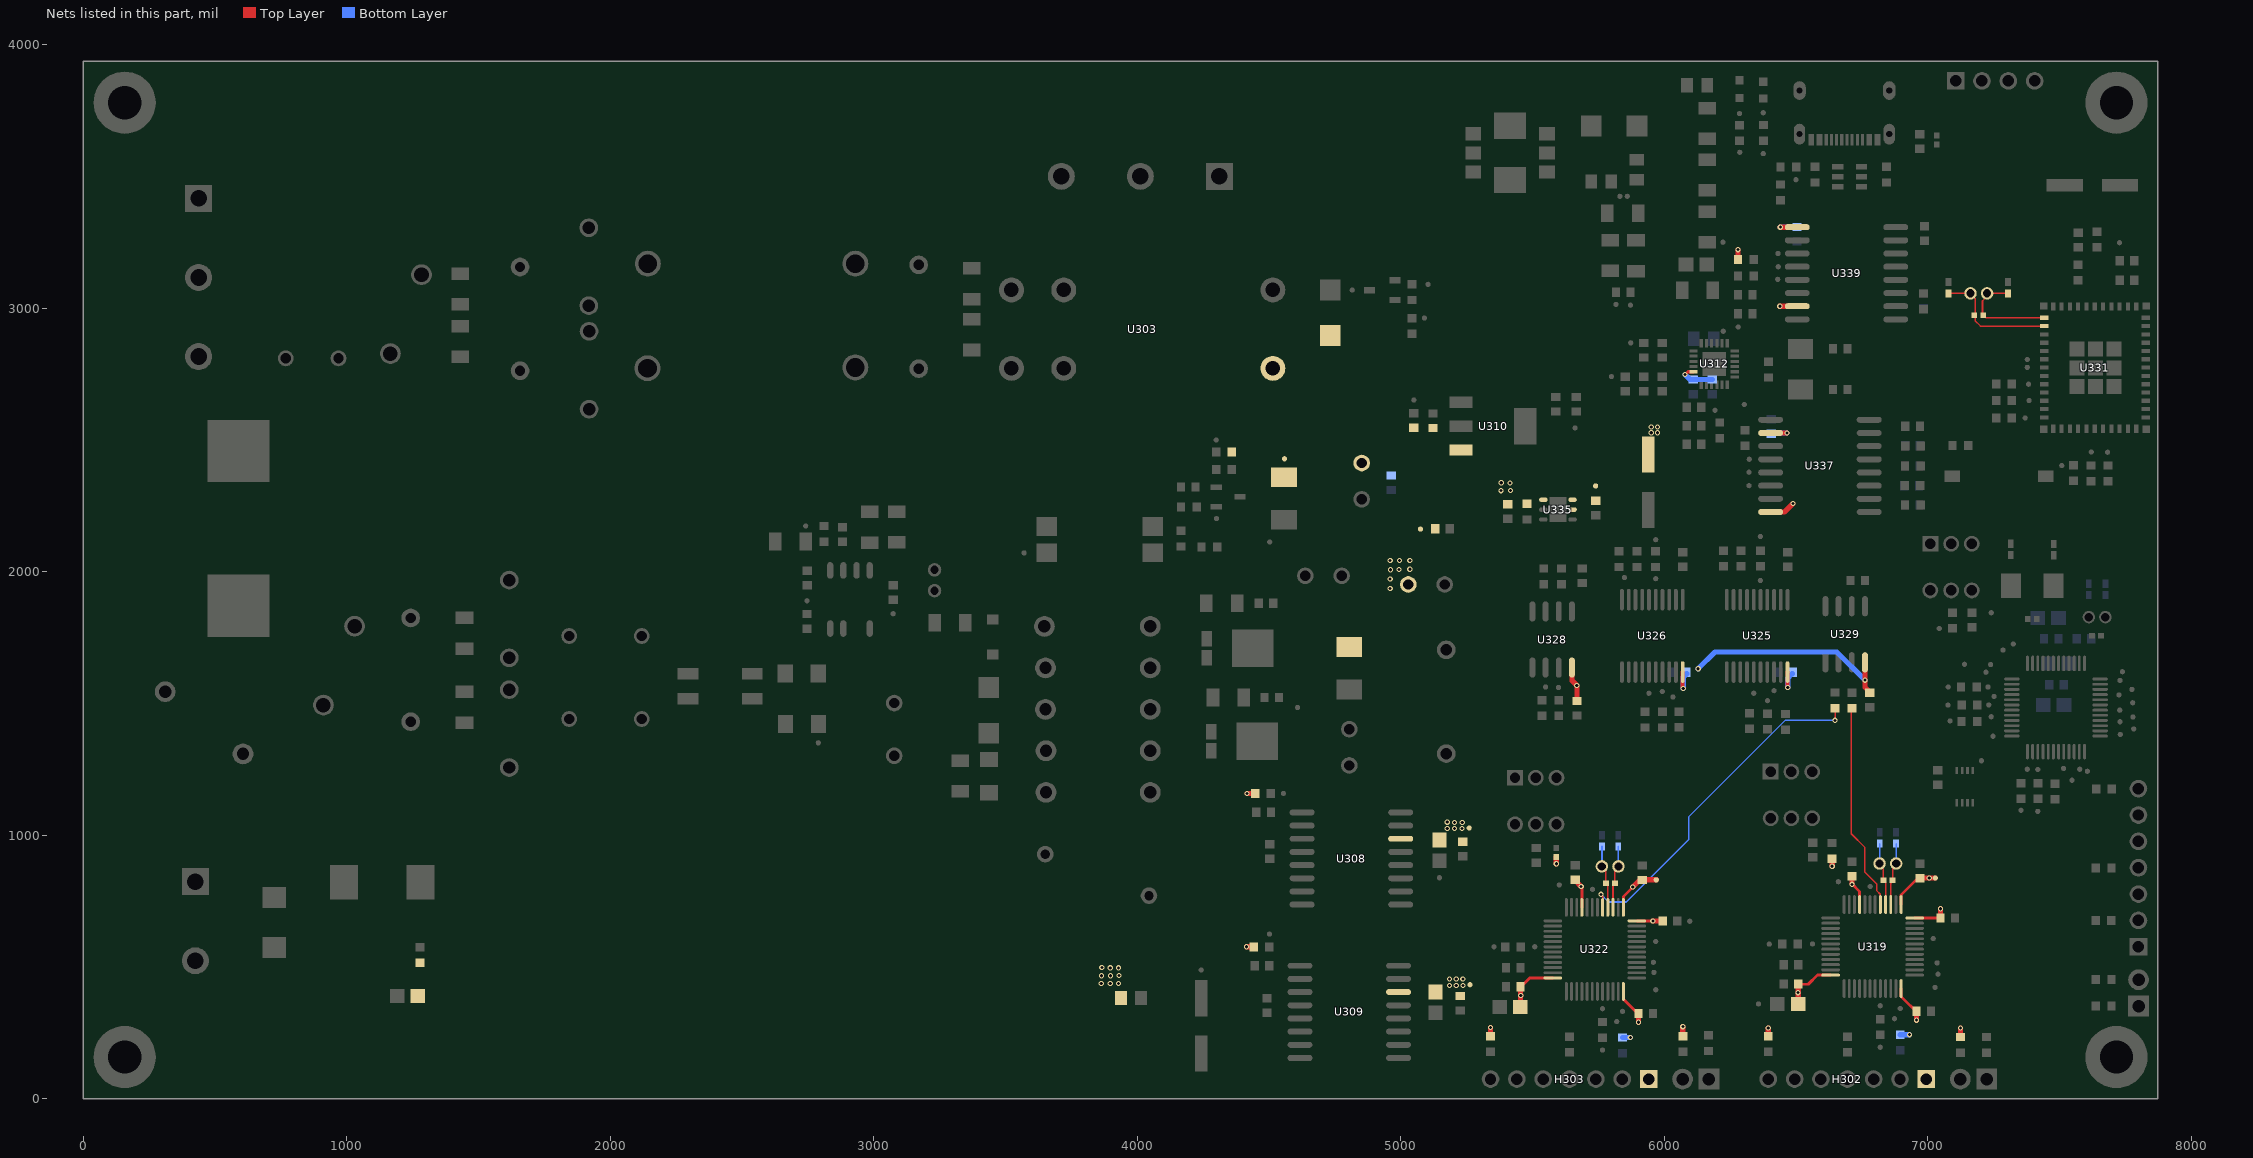
[diagram p0: the nets of this part, all layers, seen from the top]
# Altium PCB MISC84429.PcbDoc (part 5 of 5)
Units mil, origin at the board's own origin, x right, y up, seen from the top; angles counter-clockwise.
Board outline 7874.02 x 3937.01 mil, 4 copper layers (Top Layer, GND, POWER, Bottom Layer); 424 components, 202 nets, 1144 pads, 784 vias.

## Via types
v1: diameter 20, hole 12, Top Layer to Bottom Layer, tented both sides, 695 vias
v2: diameter 20, hole 12, Top Layer to Bottom Layer, 87 vias
v3: diameter 30, hole 15, Top Layer to Bottom Layer, tented both sides, 2 vias

## Nets (pads, with @x,y where several pads share a name; then routed paths per layer and width w, separated by ;. In a path a pad name is that pad's centre, name@x,y a point inside that pad or via, vN(x,y) a via of type N, cw(c..) or ccw(c..) an arc to the next point about the centre after c; other vN are vias at no path point) (continued)
VCC_3V3_HOT: C345.1 C346.1 C347.1 C414.2 C416.1 C418.1 R336.2 TP326.1 U312.17 U335.2 U335.3 U337.10 U337.16 U339.1 U339.7 | length 589.9
  Top Layer w12: v1(6079,2748) 6080,2748 6090.47,2758.47 U312.17@6111.58,2758.47
  Top Layer w20: R336.2@6280.34,3184 v1(6280.34,3221.66) ; U337.16@6403.98,2226 6457,2226 v2(6489,2258) ; U337.10@6403.98,2526 v2(6466,2526) ; v2(6439,3007) U339.7@6504.98,3007 ; v2(6441,3307) U339.1@6504.98,3307
  Bottom Layer w20: v1(6079,2748) 6098.44,2728.56 C346.1@6111,2728.56 C345.1@6183,2728.56 ; C416.1@6411,2526 v2(6466,2526) ; v2(6441,3307) C418.1@6499,3307
  other v2: 5951,2527 5975,2527 5951,2549 5975,2549
VCC_3V3_ISO_1: C324.1 C325.2 C371.1 C372.1 C373.1 C374.1 C375.2 C376.2 C390.1 H302.1 R362.2 R365.2 R366.2 R367.2 TP316.1 TP377.1 U308.14 U319.1 U319.9 U319.24 U319.36 U319.48 U325.20 | length 1009.4
  Top Layer w11: C376.2@6511,438 C376.2@6511.5,438.5 ; C376.2@6516,434 6547,434 6581.73,468.73 U319.24@6631.55,468.73 ; v1(6713,813) 6713,815 6741.79,786.21 U319.9@6741.79,736.45 ; U319.36@6899.27,417.55 6899.27,387.73 C374.1@6964,323 ; U319.1@6899.27,736.45 6899.27,772.27 C372.1@6962,835 ; U319.48@6950.45,685.27 C373.1@7047.73,685.27
  Top Layer w15: v1@6468.16,1560.84 U325.20@6468.16,1618.56
  Top Layer w20: R367.2@6395,236.66 v1(6395,268) ; v1(6508,402) v1@6508.37,402 ; C375.2@6508.37,359 v1@6508.37,402 ; C376.2@6508.37,421.37 v1@6508.37,402 ; v1(6637.57,881.43) R365.2@6637.57,910.47 ; v1@6713,815 C371.1@6713,839 ; v1(6957.44,297.56) C374.1@6957.44,331 ; 6989,837 v1(7006,837) TP377.1@7029,837 ; C373.1@7048.44,685 v1(7048.44,720.56) ; R362.2@7125,233.66 v1(7125,268)
  Bottom Layer w20: v1(6469,1560) 6468.57,1559.57 6468.57,1573.2 6468.57,1594.57 C390.1@6486,1612 ; R366.2@6896,242.66 v1(6930.66,242.66)
  other v1: 5177,1025 5204,1025 5233,1025 5204,1048 5234,1048 5177,1049
VCC_3V3_ISO_2: C330.1 C331.2 C381.1 C382.1 C383.1 C384.1 C385.2 C386.2 C392.1 C395.1 C397.1 H303.1 R370.2 R374.2 R375.2 R376.2 TP318.1 TP390.1 U309.14 U322.1 U322.9 U322.24 U322.36 U322.48 U326.20 U328.8 U329.8 | length 1945.6
  Top Layer w11: C386.2@5463,431 5489.73,457.73 U322.24@5577.55,457.73 ; U322.9@5687.79,725.45 v1@5687.79,801.79 ; U322.36@5845.27,406.55 5845.27,376.73 C384.1@5906,316 ; U322.1@5845.27,753.27 U322.1@5845.27,725.45 5845.27,766.27 v1@5881.5,802.5 ; v1(5881,803) v1@5881.5,802.5 ; v1@5882.5,803.5 v1@5881.5,802.5 ; U322.48@5896.45,674.27 v1@5953.73,674.27
  Top Layer w15: U326.20@6070.16,1618.56 6070.16,1561.84 v1@6073,1559
  Top Layer w20: R376.2@5341,236.66 v1(5341,270) ; C385.2@5454.56,367.44 v1@5454.56,392 ; C386.2@5454.56,424 v1@5454.56,392 ; v1(5455.56,391) v1@5454.56,392 ; v1(5590.95,891.05) R374.2@5590.95,916.44 ; U328.8@5650,1635.5 5650,1586 v1@5669,1567 ; C381.1@5663,830.44 5663,827 v1(5685,805) ; v1(5668,1568) v1@5669,1567 ; C395.1@5669,1517 v1@5669,1567 ; v1@5882,804 5907.44,829.44 C382.1@5917,829.44 ; v1(5902.44,289.56) C384.1@5902.44,323 ; C382.1@5927,830 TP390.1@5970,830 ; v1(5957,674) C383.1@5994.44,674 ; R370.2@6071,236.66 v1(6071,273) ; U329.8@6762,1655.5 v1(6762,1588) 6762,1561 C397.1@6779,1544
  Bottom Layer w20: R375.2@5842,231.66 v1(5871.66,231.66) ; v1(6072.56,1556.44) 6072.56,1598.56 C392.1@6086,1612 ; v1(6129,1631) 6193,1695 6655,1695 v1(6762,1588)
  other v1: 5185,429 5211,429 5237,429 5185,454 5211,454 5236,454
VCC_5V: C309.1 C311.2 C321.2 C332.2 C333.1 D301.1 F303.1 L302.2 L306.1 R318.2 R324.2 R325.2 TP306.1 U303.1 U310.3 | length 58.7
  Top Layer w20: v1(4415,576) R325.2@4442.34,576 ; v1(4417,1158) R324.2@4448.34,1158
  other v1: 3864,437 3898,437 3929,437 3865,466 3899,466 3931,467 3898,496 3929,496 3866,497 4960,1936 4960,1972 4961,2007 4994,2008 5035,2009 4960,2042 4996,2042 5035,2042
VCC_6V5: C415.2 C421.1 C422.2 L311.2 R416.1 TP428.1 U335.4
  other v2: 5381,2307 5417,2308 5415,2336 5382,2337
XTAL_8M_IN_U575: R393.1 U319.5 | length 777.3
  Top Layer w6: R393.1@6710,1468 6710,1005 6762,953 6762,859 6806,815 6806,790 6820.53,775.47 U319.5@6820.53,736.45
XTAL_8M_IN_U575_2: R395.1 U322.5 | length 1336.1
  Top Layer w6: v1(5760,775) 5766.53,768.47 U322.5@5766.53,725.45 ; v1(6648.74,1435.26) R395.1@6648.74,1481.46
  Bottom Layer w6: v1(5760,775) 5789,746 5856,746 5890,780 ; 5888,778 5890,780 ; v1@6647,1435 6459,1435 6094,1070 6094,984 5890,780
XTAL_32.768KHZ_IN_ESP32: C403.1 R402.1 U331.13 X306.2 | length 463.7
  Top Layer w6: C403.1@7078.46,3055.54 C403.1@7079,3055.54 X306.2@7150.54,3055.54 ; X306.2@7162,3050 X306.2@7173.49,3038.51 ; X306.2@7166,3051 7180,3037 7180,2952 7200.51,2931.49 U331.13@7442.09,2931.49
XTAL_32.768KHZ_IN_U575: C370.1 R360.1 U319.3 X304.1 | length 219.6
  Top Layer w6: U319.3@6859.9,736.45 6859.9,816.9 6868,825 6868,877 X304.1@6878,887
  Bottom Layer w6: X304.1@6880,906 C370.1@6880,967.54
XTAL_32.768KHZ_IN_U575_2: C380.1 R369.1 U322.3 X305.1 | length 229
  Top Layer w6: U322.3@5805.9,725.45 R369.1@5805.9,809.86 ; R369.1@5813.04,817 5813.04,867.54 X305.1@5826.5,881
  Bottom Layer w6: X305.1@5826,881.5 C380.1@5826,956.54
XTAL_32.768KHZ_OUT_ESP32: C402.2 R402.2 U331.12 X306.1 | length 375.1
  Top Layer w6: R402.2@7208.04,2973 7208.04,3027.04 X306.1@7221,3040 ; R402.2@7211.04,2973 7221.02,2962.98 U331.12@7442.09,2962.98 ; X306.1@7237.54,3055.54 C402.2@7305,3055.54
XTAL_32.768KHZ_OUT_U575: C369.2 R360.2 U319.4 X304.2 | length 211.9
  Top Layer w6: X304.2@6824,878 6832,870 6832,827 6840.21,818.79 U319.4@6840.21,736.45
  Bottom Layer w6: X304.2@6813,906 6818,911 C369.2@6818,967.54
XTAL_32.768KHZ_OUT_U575_2: C379.2 R369.2 U322.4 X305.2 | length 240
  Top Layer w6: X305.2@5763.5,881 5778.96,865.54 R369.2@5778.96,817 5786.21,809.75 U322.4@5786.21,725.45
  Bottom Layer w6: X305.2@5764,881.5 C379.2@5764,956.54
pads on no net: U304.4 U304.8 U315.2 U315.4 U315.5 U315.6 U316.1 U316.22 U316.26 U316.30 U316.31 U316.34 U316.37 U316.44 U319.2 U319.6 U319.11 U319.12 U319.13 U319.14 U319.16 U319.19 U319.20 U319.21 U319.25 U319.26 U319.27 U319.28 U319.29 U319.30 U319.31 U319.40 U319.41 U319.42 U319.43 U319.45 U319.46 U322.2 U322.6 U322.11 U322.12 U322.13 U322.14 U322.16 U322.19 U322.20 U322.21 U322.25 U322.26 U322.27 U322.28 U322.29 U322.30 U322.31 U322.40 U322.41 U322.42 U322.43 U322.45 U322.46 U325.9 U325.12 U326.9 U326.12 U331.4 U331.7 U331.19 U331.21 U331.24 U331.25 U331.26 U331.27 U331.28 U331.29 U331.32 U331.33 U331.34 U331.35 U335.5 USB301.3 USB301.9

## Polygon pours and split planes (outlines as drawn)
GND on Top Layer "Bottom Layer-No Net" (solid, remove dead copper): 87 vertices, not listed, extent 6646,304 7850,3916
GND on Top Layer "Bottom Layer-No Net" (solid, remove dead copper): 38 vertices, not listed, extent 4006.2,1049.84 4893.2,1291.84
PGND on Top Layer "Bottom Layer-No Net" (solid, remove dead copper): 18 vertices, not listed, extent 5093,1204 5285,1348
GND on Top Layer "Bottom Layer-No Net" (solid, remove dead copper): 31 vertices, not listed, extent 5089,1658 5346,2206
220V_N_OUT on Top Layer "Bottom Layer-No Net" (solid, remove dead copper): 104 vertices, not listed, extent 2868,2124 6762,3901
VCC_5V on Top Layer "Bottom Layer-No Net" (solid, remove dead copper): 75 vertices, not listed, extent 4343,1662 5297,2939
VCC_3V3_HOT on Top Layer "Bottom Layer-No Net" (solid, remove dead copper): 26 vertices, not listed, extent 5636,2225 6014,2562
VCC_6V5 on Top Layer "Bottom Layer-No Net" (solid, remove dead copper): 20 vertices, not listed, extent 5360,2238 5558,2353
VCC_6V5 on Top Layer "Bottom Layer-No Net" (solid, remove dead copper): 23 vertices, not listed, extent 4486,2301 4908,2524
VCC_3V3 on Top Layer "Bottom Layer-No Net" (solid, remove dead copper): 29 vertices, not listed, extent 5182,2424 5691,2625
NetC420_1 on Top Layer "Bottom Layer-No Net" (solid, remove dead copper): 30 vertices, not listed, extent 4356,1622 4675,2234
NetC423_2 on Top Layer "Bottom Layer-No Net" (solid, remove dead copper): 18 vertices, not listed, extent 4350,1831 4478,1934
NetC306_1 on Top Layer "Bottom Layer-No Net" (solid, remove dead copper): 34 vertices, not listed, extent 4374,1269 4889,1593
NetD310_1 on Top Layer "Bottom Layer-No Net" (solid, remove dead copper): 26 vertices, not listed, extent 4001,1623 4291,1930
NetD303_1 on Top Layer "Bottom Layer-No Net" (solid, remove dead copper): 26 vertices, not listed, extent 4005,1237 4314,1570
VCC_3V3 on Top Layer "Bottom Layer-No Net" (solid, remove dead copper, pour order 1002): 42 vertices, not listed, extent 7623,2987 7812,3506
VCC_3V3_ISO_1 on Top Layer "Bottom Layer-No Net" (solid, remove dead copper, pour order 1000): 27 vertices, not listed, extent 4950,953 5277,1061
NetC404_2 on Top Layer "Bottom Layer-No Net" (solid, remove dead copper, pour order 1000): 48 vertices, not listed, extent 6469,3617 7050,3865
NetR301_1 on Top Layer "Bottom Layer-No Net" (solid, remove dead copper, pour order 1003): 19 vertices, not listed, extent 1385,2906 1476,3038
NetR308_1 on Top Layer "Bottom Layer-No Net" (solid, remove dead copper, pour order 1005): 18 vertices, not listed, extent 1386,1515 1503,1732
NetD302_4 on Top Layer "Bottom Layer-No Net" (solid, remove dead copper, pour order 1007): 18 vertices, not listed, extent 2082,1318 2338,1542
NetD302_3 on Top Layer "Bottom Layer-No Net" (solid, remove dead copper, pour order 1008): 18 vertices, not listed, extent 2086,1583 2340,1871
NetD302_1 on Top Layer "Bottom Layer-No Net" (solid, remove dead copper, pour order 1009): 18 vertices, not listed, extent 2497,1317 2697,1543
NetD302_2 on Top Layer "Bottom Layer-No Net" (solid, remove dead copper, pour order 1010): 18 vertices, not listed, extent 2497,1571 2696,1697
NetC313_1 on Top Layer "Bottom Layer-No Net" (solid, remove dead copper, pour order 1012): 18 vertices, not listed, extent 3280,1255 3507,1431
NetD305_2 on Top Layer "Bottom Layer-No Net" (solid, remove dead copper, pour order 1013): 42 vertices, not listed, extent 2959,1432 3696,1818
NetD304_2 on Top Layer "Bottom Layer-No Net" (solid, remove dead copper, pour order 1014): 26 vertices, not listed, extent 3414,1579 3693,1712
NetD304_1 on Top Layer "Bottom Layer-No Net" (solid, remove dead copper, pour order 1015): 18 vertices, not listed, extent 3322,1764 3492,1876
NetC314_1 on Top Layer "Bottom Layer-No Net" (solid, remove dead copper, pour order 1016): 37 vertices, not listed, extent 2870,1749 3258,1953
NetR319_2 on Top Layer "Bottom Layer-No Net" (solid, remove dead copper, pour order 1017): 26 vertices, not listed, extent 2949,1973 3128,2136
NetC318_2 on Top Layer "Bottom Layer-No Net" (solid, remove dead copper, pour order 1018): 33 vertices, not listed, extent 2717,1971 2903,2186
VBUS on Top Layer "Bottom Layer-No Net" (solid, remove dead copper, pour order 1019): 18 vertices, not listed, extent 2558,2068 2653,2174
NetR303_1 on Top Layer "Bottom Layer-No Net" (solid, remove dead copper, pour order 1021): 18 vertices, not listed, extent 3317,2932 3430,3059
220V_RELAY_IN on Top Layer "Bottom Layer-No Net" (solid, remove dead copper, pour order 1022): 30 vertices, not listed, extent 2859,2579 3594,3122
NetC306_2 on Top Layer "Bottom Layer-No Net" (solid, remove dead copper, pour order 1024): 18 vertices, not listed, extent 4378,1477 4501,1569
NetD306_2 on Top Layer "Bottom Layer-No Net" (solid, remove dead copper, pour order 1026): 17 vertices, not listed, extent 360,723 1063,979
NetC322_1 on Top Layer "Bottom Layer-No Net" (solid, remove dead copper, pour order 1027): 61 vertices, not listed, extent 3990,310 4678,1024
NetD306_1 on Top Layer "Bottom Layer-No Net" (solid, remove dead copper, pour order 1029): 18 vertices, not listed, extent 1203,558 1437,907
VCC_5V on Top Layer "Bottom Layer-No Net" (solid, remove dead copper, pour order 1030): 18 vertices, not listed, extent 1242,223 3960,529
VCC_3V3_ISO_2 on Top Layer "Bottom Layer-No Net" (solid, remove dead copper, pour order 1032): 23 vertices, not listed, extent 4943,376 5279,466
AGND on Top Layer "Bottom Layer-No Net" (solid, remove dead copper, pour order 1000): 25 vertices, not listed, extent 2757,1457 3211,1685
AGND on Top Layer "Bottom Layer-No Net" (solid, remove dead copper, pour order 1001): 26 vertices, not listed, extent 2792,2129 3698,2284
AGND on Top Layer "Bottom Layer-No Net" (solid, remove dead copper, pour order 1002): 38 vertices, not listed, extent 3053,1750 3694,2037
VBUS on Top Layer "Bottom Layer-No Net" (solid, remove dead copper, pour order 1003): 26 vertices, not listed, extent 2757,1015 3698,1474
AGND on Top Layer "Bottom Layer-No Net" (solid, remove dead copper, pour order 1004): 20 vertices, not listed, extent 2724,871 3688,1140
GND on Top Layer "Bottom Layer-No Net" (solid, remove dead copper, pour order 1005): 36 vertices, not listed, extent 351,35 4666,617
GND on Top Layer "Bottom Layer-No Net" (solid, remove dead copper, pour order 1006): 23 vertices, not listed, extent 4416,703 4673,948
GND on Top Layer "Bottom Layer-No Net" (solid, remove dead copper, pour order 1008): 41 vertices, not listed, extent 4934,2584 5709,3138
GND on Top Layer "Bottom Layer-No Net" (solid, remove dead copper, pour order 1010): 18 vertices, not listed, extent 7429,3302 7599,3557
GND on Top Layer "Bottom Layer-No Net" (solid, remove dead copper, pour order 1011): 7769,3177 7769,3043.85 7779,3033.85 7796,3033.85 7840.85,3033.85 7851,3044 7851,3057 7851,3216 7842,3225 7837,3230 7826,3230 7781,3230 7777,3226 7769,3218 7769,3177
PGND on Top Layer "Bottom Layer-No Net" (solid, remove dead copper, pour order 1012): 41 vertices, not listed, extent 4949,675 5333,1152
PGND on Top Layer "Bottom Layer-No Net" (solid, remove dead copper, pour order 1013): 50 vertices, not listed, extent 4943,26 5403,547
PGND on Top Layer "Bottom Layer-No Net" (solid, remove dead copper, pour order 1014): 49 vertices, not listed, extent 5395,778 5981,1300
PGND on Top Layer "Bottom Layer-No Net" (solid, remove dead copper, pour order 1015): 46 vertices, not listed, extent 6740,782 7025,1446
NetC302_1 on Top Layer "Bottom Layer-No Net" (solid, remove dead copper, pour order 1031): 26 vertices, not listed, extent 364,3359 3782,3891
NetC307_1 on Top Layer "Bottom Layer-No Net" (solid, remove dead copper, pour order 1004): 34 vertices, not listed, extent 545,1221 1881,1536
NetC305_2 on Top Layer "Bottom Layer-No Net" (solid, remove dead copper, pour order 1006): 38 vertices, not listed, extent 430,1721 1903,2147
NetC301_2 on Top Layer "Bottom Layer-No Net" (solid, remove dead copper, pour order 1001): 30 vertices, not listed, extent 934,2336 2203,2880
NetF301_1 on Top Layer "Bottom Layer-No Net" (solid, remove dead copper, pour order 1000): 19 vertices, not listed, extent 383,2323 803,2871
NetC301_1 on Top Layer "Bottom Layer-No Net" (solid, remove dead copper, pour order 1002): 44 vertices, not listed, extent 42,1497 2206,3437
no net on Keep-Out Layer (none): 29 vertices, not listed, extent 247.49,1601.49 1330.51,3040.51
GND on Bottom Layer "Bottom Layer-No Net" (solid, remove dead copper): 30 vertices, not listed, extent 7133,324 7688,1208
GND on Bottom Layer "Bottom Layer-No Net" (solid, remove dead copper): 78 vertices, not listed, extent 6867,1636 7755,2937
GND on Bottom Layer "Bottom Layer-No Net" (solid, remove dead copper): 100 vertices, not listed, extent 6384,2285 7850,3916
220V_N_OUT on Bottom Layer "Bottom Layer-No Net" (solid, remove dead copper): 26 vertices, not listed, extent 5348,2118 5783,2376
GND on Bottom Layer "Bottom Layer-No Net" (solid, remove dead copper): 38 vertices, not listed, extent 4713,2564 5709,3143
GND on Bottom Layer "Bottom Layer-No Net" (solid, remove dead copper): 27 vertices, not listed, extent 5131,1663 5343,2206
220V_N_OUT on Bottom Layer "Bottom Layer-No Net" (solid, remove dead copper): 55 vertices, not listed, extent 4005,1551 5020,2325
VCC_6V5 on Bottom Layer "Bottom Layer-No Net" (solid, remove dead copper): 29 vertices, not listed, extent 4813,2290 5440,2476
VCC_5V on Bottom Layer "Bottom Layer-No Net" (solid, remove dead copper): 61 vertices, not listed, extent 3849,332 5063,2066
NetL307_1 on Bottom Layer "Bottom Layer-No Net" (solid, remove dead copper): 23 vertices, not listed, extent 6145,2753 6248,2919
NetC301_2 on Bottom Layer "Bottom Layer-No Net" (solid, remove dead copper, pour order 1001): 30 vertices, not listed, extent 934,2336 2203,2880
NetF301_1 on Bottom Layer "Bottom Layer-No Net" (solid, remove dead copper, pour order 1000): 19 vertices, not listed, extent 383,2323 803,2871
NetC301_1 on Bottom Layer "Bottom Layer-No Net" (solid, remove dead copper, pour order 1002): 44 vertices, not listed, extent 42,1497 2206,3437
220V_N_OUT on Bottom Layer "Bottom Layer-No Net" (solid, remove dead copper, pour order 1004): 74 vertices, not listed, extent 2880,2666 6135,3900
VBUS on Bottom Layer "Bottom Layer-No Net" (solid, remove dead copper, pour order 1033): 26 vertices, not listed, extent 2516,1193 3127,2170
AGND on Bottom Layer "Bottom Layer-No Net" (solid, remove dead copper, pour order 1016): 49 vertices, not listed, extent 2715,869 3697,2284
GND on Bottom Layer "Bottom Layer-No Net" (solid, remove dead copper, pour order 1017): 82 vertices, not listed, extent 345,34 4667,1125
PGND on Bottom Layer "Bottom Layer-No Net" (solid, remove dead copper, pour order 1019): 50 vertices, not listed, extent 4951,27 7300,1690
NetC302_1 on Bottom Layer "Bottom Layer-No Net" (solid, remove dead copper, pour order 1031): 26 vertices, not listed, extent 364,3359 3782,3891
VCC_3V3_ISO_2 on POWER "Bottom Layer-No Net" (solid, remove dead copper): 39 vertices, not listed, extent 5113,23 6227,1650
GND on POWER "Bottom Layer-No Net" (solid, remove dead copper): 75 vertices, not listed, extent 345,34 5711,3150
VCC_3V3 on POWER "Bottom Layer-No Net" (solid, remove dead copper): 53 vertices, not listed, extent 5346,427 7850,3443
VCC_3V3_HOT on POWER "Bottom Layer-No Net" (solid, remove dead copper): 42 vertices, not listed, extent 5910,2241 6639,3321
NetL307_1 on POWER "Bottom Layer-No Net" (solid, remove dead copper, pour order 1008): 18 vertices, not listed, extent 6148,2731 6277,2845
220V_N_OUT on POWER "Bottom Layer-No Net" (solid, remove dead copper, pour order 1007): 41 vertices, not listed, extent 3917,2666 6226,3904
VCC_3V3_ISO_1 on POWER "Bottom Layer-No Net" (solid, remove dead copper, pour order 1005): 76 vertices, not listed, extent 4999,24 7306,1874
AGND on POWER "Bottom Layer-No Net" (solid, remove dead copper, pour order 1020): 2714,2256 2714,905 2746,873 2755,864 2761,864 3638,864 3699,925 3700,926 3700,928 3700,2261 3676,2285 3674,2285 2743,2285 2714,2256
NetC302_1 on POWER "Bottom Layer-No Net" (solid, remove dead copper, pour order 1036): 68 vertices, not listed, extent 364,1510 3785,3890
220V_N_OUT on GND "Bottom Layer-No Net" (solid, remove dead copper): 69 vertices, not listed, extent 3917,1941 6769,3907
PGND on GND "Bottom Layer-No Net" (solid, remove dead copper): 24 vertices, not listed, extent 4949,21 7306,1696
GND on GND "Bottom Layer-No Net" (solid, remove dead copper): 143 vertices, not listed, extent 345,34 7852,3907
AGND on GND "Bottom Layer-No Net" (solid, remove dead copper, pour order 1021): 19 vertices, not listed, extent 2714,864 3700,2285
NetC301_1 on GND "Bottom Layer-No Net" (solid, remove dead copper, pour order 1002): 44 vertices, not listed, extent 44,1495 2208,3435
NetF301_1 on GND "Bottom Layer-No Net" (solid, remove dead copper, pour order 1000): 19 vertices, not listed, extent 383,2324 803,2872
NetC301_2 on GND "Bottom Layer-No Net" (solid, remove dead copper, pour order 1001): 30 vertices, not listed, extent 934,2336 2203,2880
NetC302_1 on GND "Bottom Layer-No Net" (solid, remove dead copper, pour order 1031): 26 vertices, not listed, extent 364,3359 3782,3891

## Keep-outs
Keep-Out Layer:
  lines w5: 250,2850 250,2902 386,3038 1320,3038 1328,3030 1328,2949 1317,2938 437,2938 348,2849 348,1822 459,1711 1309,1711 1317,1703 1317,1615 1306,1604 405,1604 250,1759 250,2852 ; 121,1034 121,1168 140,1187 1513,1187 1900,800 3674,800 3740,866 3740,2282 3696,2326 2666,2326 2379,2613 2379,3649 2402,3672 2709,3672 2734,3647 2734,2671 2860,2545 3825,2545 3970,2400 3970,739 3843,612 1769,612 1372,1009 146,1009 121,1034
  lines w6: 0,0 0,3937.01 7874.02,3937.01 7874.02,0 0,0

## Silkscreen, mask and mechanical layers (free items; w line width, h text height)
Top Overlay:
  text "TDI" at 7322,3715 h50 r90
  text "TMS" at 7426,3708 h50 r90
  text "TDO" at 7125,3707 h50 r90
  text "TCK" at 7220,3707 h50 r90
  text "High voltage danger" at 3222,3613 h80
  text "PE" at 646,3419 h50
  text "PE" at 3681,3257 h60
  text "L_O" at 3983,3254 h60
  text "N_O" at 4282,3247 h60
  text "L" at 643,3117 h50
  text "High voltage danger" at 822,3079 h80 r90
  text "N" at 640,2794 h50
  text "High voltage danger" at 4658,2726 h80
  text "5V" at 648,846 h60
  text "GND" at 641,428 h60
  text "USE ISOLATOR!" at 7576,366 h50 r90
  text "DEBUG" at 311,236 h100
Bottom Overlay:
  text "TX" at 7721,1157 h50
  text "RX" at 7724,1063 h50
  text "NST" at 7724,968 h50
  text "CLK" at 7725,861 h50
  text "GNDB" at 7739,759 h50
  text "DIO" at 7713,661 h50
  text "3V3" at 7714,558 h50
  text "3V3" at 7711,438 h50
  text "BOOT" at 7717,336 h50
  text "3V3" at 7028,165 h50 r90
  text "DIO" at 6975,163 h50 r90
  text "TX" at 6419,160 h50 r90
  text "CLK" at 6716,157 h50 r90
  text "3V3" at 7101,157 h50 r270
  text "NST" at 6613,156 h50 r90
  text "TX2" at 5358,154 h50 r90
  text "RX2" at 5457,153 h50 r90
  text "RX" at 6522,152 h50 r90
  text "GNDC" at 6809,152 h50 r90
  text "CLK2" at 5659,151 h50 r90
  text "3V3" at 5977,151 h50 r90
  text "3V3" at 6052,151 h50 r270
  text "BOOT" at 7208,151 h50 r270
  text "NST2" at 5559,150 h50 r90
  text "DIO2" at 5926,149 h50 r90
  text "GNDC" at 5759,145 h50 r90
  text "BOOT2" at 6152,143 h50 r270
Bottom Solder:
  region: 2885,3151 2914,3122 3388,3122 3497,3231 4065,3231 4107,3273 4107,3539 4085,3561 3962,3561 3930,3529 3930,3455 3879,3404 2914,3404 2885,3375
  region: 1225,2873 1254,2844 1657,2844 1719,2782 1808,2693 1971,2693 2074,2796 2108,2830 2179,2830 2186,2823 2203,2806 2203,2725 2203,2465 2194,2456 2074,2336 1117,2336 1021,2432 934,2519 934,2814 934,2836 946,2848 978,2880 1218,2880
  region: 790,2856 803,2843 803,2783 803,2380 763,2340 746,2323 419,2323 408,2334 383,2359 383,2797 383,2834 383,2835 383,2844 398,2859 410,2871 775,2871
  region: 2159,3424 2206,3377 2206,3162 2206,3135 2197,3126 2176,3105 2084,3105 2020,3169 1958,3231 1808,3231 1746,3169 1677,3100 1331,3100 1317,3086 1297,3066 354,3066 288,3000 223,2935 223,2198 223,1750 260,1713 363,1610 363,1527 363,1517 359,1513 343,1497 96,1497 68,1525 42,1551 42,3093 204,3255 574,3255 643,3324 756,3437 2146,3437
  region: 3681,3802 3782,3701 3782,3519 3782,3475 3778,3471 3758,3451 3517,3451 3472,3496 3259,3709 839,3709 514,3384 489,3359 388,3359 382,3365 364,3383 364,3522 364,3523 364,3715 395,3746 540,3891 3592,3891